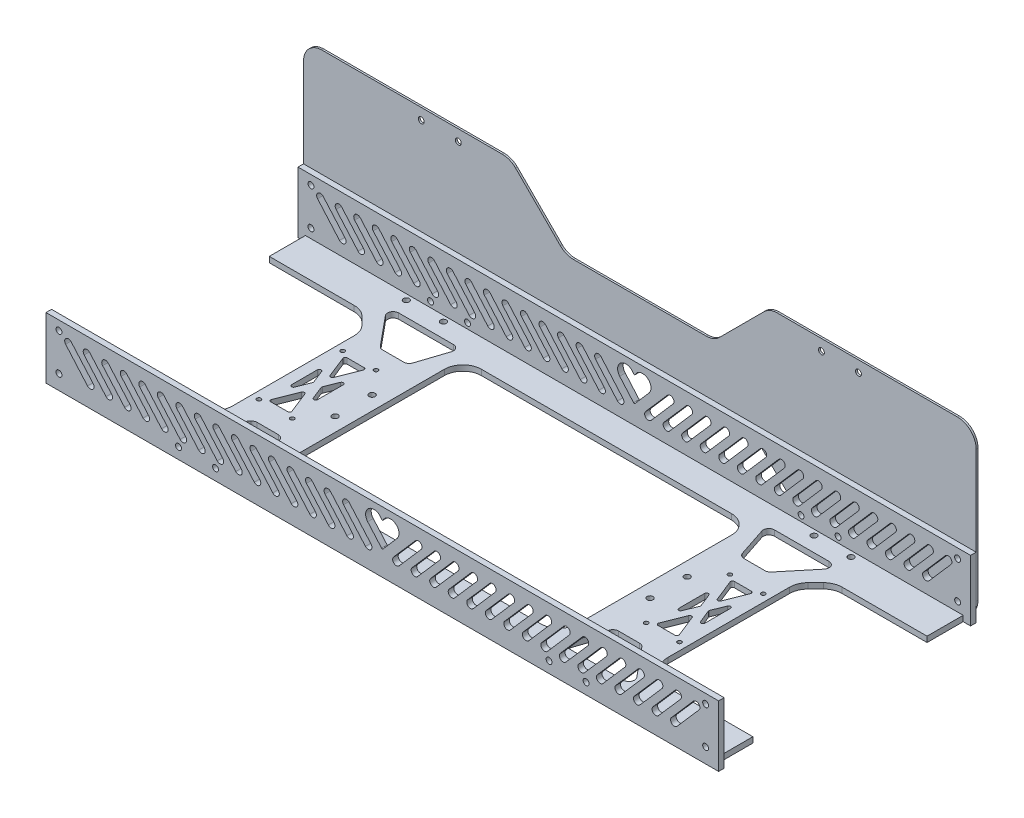
from build123d import *

# Parameters (mm, degrees)
SKETCH_1_W          = 355
SKETCH_1_H          = 133
SKETCH_1_R          = 1.6
EXTRUDE_1_DEPTH     = 3
SKETCH_2_W          = 363
SKETCH_2_H          = 33
SKETCH_2_R          = 1.6
EXTRUDE_2_DEPTH     = 3
SKETCH_3_R          = 1.6
SKETCH_3_R_2        = 1.1
CUT_EXTRUDE_1_DEPTH = 10
FILLET_1_R          = 10
CUT_EXTRUDE_2_DEPTH = 231.98105983
CUT_EXTRUDE_3_DEPTH = 10
SKETCH_7_R          = 1.6
EXTRUDE_3_DEPTH     = 1
FILLET_2_R          = 10


with BuildPart() as part:
    # 草图1 → 凸台-拉伸1 (new body)
    with BuildSketch(Plane(origin=(0, 0, 0), x_dir=(1, 0, 0), z_dir=(0, 1, 0))):
        Rectangle(SKETCH_1_W, SKETCH_1_H)
        with Locations(Location((-120, -63.5, 0), (0, 0, 270))):
            Circle(SKETCH_1_R, mode=Mode.SUBTRACT)
        with Locations(Location((120, -63.5, 0), (0, 0, 90))):
            Circle(SKETCH_1_R, mode=Mode.SUBTRACT)
        with Locations(Location((-100, -63.5, 0), (0, 0, 270))):
            Circle(SKETCH_1_R, mode=Mode.SUBTRACT)
        with Locations(Location((100, -63.5, 0), (0, 0, 90))):
            Circle(SKETCH_1_R, mode=Mode.SUBTRACT)
        with Locations(Location((100, 63.5, 0), (0, 0, 270))):
            Circle(SKETCH_1_R, mode=Mode.SUBTRACT)
        with Locations(Location((-100, 63.5, 0), (0, 0, 90))):
            Circle(SKETCH_1_R, mode=Mode.SUBTRACT)
        with Locations(Location((120, 63.5, 0), (0, 0, 270))):
            Circle(SKETCH_1_R, mode=Mode.SUBTRACT)
        with Locations(Location((-120, 63.5, 0), (0, 0, 90))):
            Circle(SKETCH_1_R, mode=Mode.SUBTRACT)
    extrude(amount=EXTRUDE_1_DEPTH)

    # 草图3 → 切除-拉伸1 (cut)
    with BuildSketch(Plane(origin=(0, 3, 0), x_dir=(1, 0, 0), z_dir=(0, 1, 0))):
        with Locations(Location((-85, 10, 0), (0, 0, 270))):
            Circle(SKETCH_3_R)
        with Locations(Location((-85, -10, 0), (0, 0, 270))):
            Circle(SKETCH_3_R)
        with Locations(Location((85, -10, 0), (0, 0, 90))):
            Circle(SKETCH_3_R)
        with Locations(Location((85, 10, 0), (0, 0, 90))):
            Circle(SKETCH_3_R)
        with Locations(Location((-113.5, 22.6, 0), (0, 0, 270))):
            Circle(SKETCH_3_R_2)
        with Locations(Location((-95.5, 22.6, 0), (0, 0, 270))):
            Circle(SKETCH_3_R_2)
        with Locations(Location((-113.5, -22.6, 0), (0, 0, 270))):
            Circle(SKETCH_3_R_2)
        with Locations(Location((-95.5, -22.6, 0), (0, 0, 270))):
            Circle(SKETCH_3_R_2)
        with Locations(Location((95.5, -22.6, 0), (0, 0, 90))):
            Circle(SKETCH_3_R_2)
        with Locations(Location((113.5, -22.6, 0), (0, 0, 90))):
            Circle(SKETCH_3_R_2)
        with Locations(Location((95.5, 22.6, 0), (0, 0, 90))):
            Circle(SKETCH_3_R_2)
        with Locations(Location((113.5, 22.6, 0), (0, 0, 90))):
            Circle(SKETCH_3_R_2)
        Polygon((-177.5, 47), (-127.5, 47), (-117.5, 37), (-117.5, -37), (-127.5, -47), (-177.5, -47), align=None)
        Polygon((177.5, 47), (127.5, 47), (117.5, 37), (117.5, -37), (127.5, -47), (177.5, -47), align=None)
        with BuildLine():
            Line((-67.5, -51.5), (67.5, -51.5))
            ThreePointArc((67.5, -51.5), (74.571067812, -48.571067812), (77.5, -41.5))
            Line((77.5, -41.5), (77.5, 41.5))
            ThreePointArc((77.5, 41.5), (74.571067812, 48.571067812), (67.5, 51.5))
            Line((67.5, 51.5), (-67.5, 51.5))
            ThreePointArc((-67.5, 51.5), (-74.571067812, 48.571067812), (-77.5, 41.5))
            Line((-77.5, 41.5), (-77.5, -41.5))
            ThreePointArc((-77.5, -41.5), (-74.571067812, -48.571067812), (-67.5, -51.5))
        make_face()
    extrude(amount=-CUT_EXTRUDE_1_DEPTH, mode=Mode.SUBTRACT)

    # 圆角1
    fillet_1_edges = [part.edges().sort_by_distance(p)[0] for p in [
        (127.5, 1.5, 47),
        (117.5, 1.5, 37),
        (117.5, 1.5, -37),
        (127.5, 1.5, -47),
        (-127.5, 1.5, -47),
        (-117.5, 1.5, -37),
        (-117.5, 1.5, 37),
        (-127.5, 1.5, 47),
    ]]
    fillet(fillet_1_edges, radius=FILLET_1_R)

    # 草图6 → 切除-拉伸3 (cut)
    with BuildSketch(Plane(origin=(0, 3, 0), x_dir=(1, 0, 0), z_dir=(0, 1, 0))):
        with BuildLine():
            Line((-109.076179073, -20.6), (-99.923820927, -20.6))
            ThreePointArc((-99.923820927, -20.6), (-99.096181899, -20.161260758), (-98.99477831, -19.230027276))
            Line((-98.99477831, -19.230027276), (-103.570957383, -7.73873316))
            ThreePointArc((-103.570957383, -7.73873316), (-104.5, -7.108705884), (-105.429042617, -7.73873316))
            Line((-105.429042617, -7.73873316), (-110.00522169, -19.230027276))
            ThreePointArc((-110.00522169, -19.230027276), (-109.903818101, -20.161260758), (-109.076179073, -20.6))
        make_face()
        with BuildLine():
            Line((-111.5, -6.957960783), (-111.5, 6.957960783))
            ThreePointArc((-111.5, 6.957960783), (-110.688357882, 7.94006124), (-109.570957383, 7.327933506))
            Line((-109.570957383, 7.327933506), (-106.800088045, 0.369972724))
            ThreePointArc((-106.800088045, 0.369972724), (-106.729130662, 0), (-106.800088045, -0.369972724))
            Line((-106.800088045, -0.369972724), (-109.570957383, -7.327933506))
            ThreePointArc((-109.570957383, -7.327933506), (-110.688357882, -7.94006124), (-111.5, -6.957960783))
        make_face()
        with BuildLine():
            Line((-103.570957383, 7.73873316), (-98.99477831, 19.230027276))
            ThreePointArc((-98.99477831, 19.230027276), (-99.096181899, 20.161260758), (-99.923820927, 20.6))
            Line((-99.923820927, 20.6), (-109.076179073, 20.6))
            ThreePointArc((-109.076179073, 20.6), (-109.903818101, 20.161260758), (-110.00522169, 19.230027276))
            Line((-110.00522169, 19.230027276), (-105.429042617, 7.73873316))
            ThreePointArc((-105.429042617, 7.73873316), (-104.5, 7.108705884), (-103.570957383, 7.73873316))
        make_face()
        with BuildLine():
            Line((-102.199911955, 0.369972724), (-99.429042617, 7.327933506))
            ThreePointArc((-99.429042617, 7.327933506), (-98.311642118, 7.94006124), (-97.5, 6.957960783))
            Line((-97.5, 6.957960783), (-97.5, -6.957960783))
            ThreePointArc((-97.5, -6.957960783), (-98.311642118, -7.94006124), (-99.429042617, -7.327933506))
            Line((-99.429042617, -7.327933506), (-102.199911955, -0.369972724))
            ThreePointArc((-102.199911955, -0.369972724), (-102.270869338, 0), (-102.199911955, 0.369972724))
        make_face()
        with BuildLine():
            Line((-118.443155104, 50.589304353), (-105.520807103, 34.947168729))
            ThreePointArc((-105.520807103, 34.947168729), (-104.486227323, 34.143818785), (-103.207964232, 33.857864376))
            Line((-103.207964232, 33.857864376), (-91.792035768, 33.857864376))
            ThreePointArc((-91.792035768, 33.857864376), (-90.033188953, 34.427543846), (-88.942328085, 35.920225789))
            Line((-88.942328085, 35.920225789), (-83.795600214, 51.562361412))
            ThreePointArc((-83.795600214, 51.562361412), (-84.214987367, 54.258846815), (-86.645307897, 55.5))
            Line((-86.645307897, 55.5), (-116.130312233, 55.5))
            ThreePointArc((-116.130312233, 55.5), (-118.844357824, 53.778263091), (-118.443155104, 50.589304353))
        make_face()
        with BuildLine():
            Line((-103.207964232, -33.857864376), (-91.792035768, -33.857864376))
            ThreePointArc((-91.792035768, -33.857864376), (-90.033188953, -34.427543846), (-88.942328085, -35.920225789))
            Line((-88.942328085, -35.920225789), (-83.795600214, -51.562361412))
            ThreePointArc((-83.795600214, -51.562361412), (-84.214987367, -54.258846815), (-86.645307897, -55.5))
            Line((-86.645307897, -55.5), (-116.130312233, -55.5))
            ThreePointArc((-116.130312233, -55.5), (-118.844357824, -53.778263091), (-118.443155104, -50.589304353))
            Line((-118.443155104, -50.589304353), (-105.520807103, -34.947168729))
            ThreePointArc((-105.520807103, -34.947168729), (-104.486227323, -34.143818785), (-103.207964232, -33.857864376))
        make_face()
        with BuildLine():
            Line((118.443155104, -50.589304353), (105.520807103, -34.947168729))
            ThreePointArc((105.520807103, -34.947168729), (104.486227323, -34.143818785), (103.207964232, -33.857864376))
            Line((103.207964232, -33.857864376), (91.792035768, -33.857864376))
            ThreePointArc((91.792035768, -33.857864376), (90.033188953, -34.427543846), (88.942328085, -35.920225789))
            Line((88.942328085, -35.920225789), (83.795600214, -51.562361412))
            ThreePointArc((83.795600214, -51.562361412), (84.214987367, -54.258846815), (86.645307897, -55.5))
            Line((86.645307897, -55.5), (116.130312233, -55.5))
            ThreePointArc((116.130312233, -55.5), (118.844357824, -53.778263091), (118.443155104, -50.589304353))
        make_face()
        with BuildLine():
            Line((86.645307897, 55.5), (116.130312233, 55.5))
            ThreePointArc((116.130312233, 55.5), (118.844357824, 53.778263091), (118.443155104, 50.589304353))
            Line((118.443155104, 50.589304353), (105.520807103, 34.947168729))
            ThreePointArc((105.520807103, 34.947168729), (104.486227323, 34.143818785), (103.207964232, 33.857864376))
            Line((103.207964232, 33.857864376), (91.792035768, 33.857864376))
            ThreePointArc((91.792035768, 33.857864376), (90.033188953, 34.427543846), (88.942328085, 35.920225789))
            Line((88.942328085, 35.920225789), (83.795600214, 51.562361412))
            ThreePointArc((83.795600214, 51.562361412), (84.214987367, 54.258846815), (86.645307897, 55.5))
        make_face()
        with BuildLine():
            Line((103.570957383, -7.73873316), (98.99477831, -19.230027276))
            ThreePointArc((98.99477831, -19.230027276), (99.096181899, -20.161260758), (99.923820927, -20.6))
            Line((99.923820927, -20.6), (109.076179073, -20.6))
            ThreePointArc((109.076179073, -20.6), (109.903818101, -20.161260758), (110.00522169, -19.230027276))
            Line((110.00522169, -19.230027276), (105.429042617, -7.73873316))
            ThreePointArc((105.429042617, -7.73873316), (104.5, -7.108705884), (103.570957383, -7.73873316))
        make_face()
        with BuildLine():
            Line((97.5, -6.957960783), (97.5, 6.957960783))
            ThreePointArc((97.5, 6.957960783), (98.311642118, 7.94006124), (99.429042617, 7.327933506))
            Line((99.429042617, 7.327933506), (102.199911955, 0.369972724))
            ThreePointArc((102.199911955, 0.369972724), (102.270869338, 0), (102.199911955, -0.369972724))
            Line((102.199911955, -0.369972724), (99.429042617, -7.327933506))
            ThreePointArc((99.429042617, -7.327933506), (98.311642118, -7.94006124), (97.5, -6.957960783))
        make_face()
        with BuildLine():
            Line((109.076179073, 20.6), (99.923820927, 20.6))
            ThreePointArc((99.923820927, 20.6), (99.096181899, 20.161260758), (98.99477831, 19.230027276))
            Line((98.99477831, 19.230027276), (103.570957383, 7.73873316))
            ThreePointArc((103.570957383, 7.73873316), (104.5, 7.108705884), (105.429042617, 7.73873316))
            Line((105.429042617, 7.73873316), (110.00522169, 19.230027276))
            ThreePointArc((110.00522169, 19.230027276), (109.903818101, 20.161260758), (109.076179073, 20.6))
        make_face()
        with BuildLine():
            Line((109.570957383, -7.327933506), (106.800088045, -0.369972724))
            ThreePointArc((106.800088045, -0.369972724), (106.729130662, 0), (106.800088045, 0.369972724))
            Line((106.800088045, 0.369972724), (109.570957383, 7.327933506))
            ThreePointArc((109.570957383, 7.327933506), (110.688357882, 7.94006124), (111.5, 6.957960783))
            Line((111.5, 6.957960783), (111.5, -6.957960783))
            ThreePointArc((111.5, -6.957960783), (110.688357882, -7.94006124), (109.570957383, -7.327933506))
        make_face()
    extrude(amount=-CUT_EXTRUDE_3_DEPTH, mode=Mode.SUBTRACT)


with BuildPart() as body_2:
    # 草图2 → 凸台-拉伸2 (new body)
    with BuildSketch(Plane.XY.offset(66.5)):
        with Locations((0, 16.5)):
            Rectangle(SKETCH_2_W, SKETCH_2_H)
        with Locations((-174.5, 28)):
            Circle(SKETCH_2_R, mode=Mode.SUBTRACT)
        with Locations(Location((174.5, 28, 0), (0, 0, 180))):
            Circle(SKETCH_2_R, mode=Mode.SUBTRACT)
        with Locations((-174.5, 8)):
            Circle(SKETCH_2_R, mode=Mode.SUBTRACT)
        with Locations(Location((174.5, 8, 0), (0, 0, 180))):
            Circle(SKETCH_2_R, mode=Mode.SUBTRACT)
        with Locations((-110, 6)):
            Circle(SKETCH_2_R, mode=Mode.SUBTRACT)
        with Locations(Location((110, 6, 0), (0, 0, 180))):
            Circle(SKETCH_2_R, mode=Mode.SUBTRACT)
        with Locations((-90, 6)):
            Circle(SKETCH_2_R, mode=Mode.SUBTRACT)
        with Locations(Location((90, 6, 0), (0, 0, 180))):
            Circle(SKETCH_2_R, mode=Mode.SUBTRACT)
    extrude(amount=EXTRUDE_2_DEPTH)


with BuildPart() as body_3:
    # 镜向1: mirrored copy
    add(body_2.part.mirror(Plane.XY))


with BuildPart() as cut_extrude_2_tool:
    # 草图4 → 切除-拉伸2 (new, through all)
    with BuildSketch(Plane.XY.offset(69.5)):
        with BuildLine():
            Line((-167.910958904, 26.095890411), (-156.075342466, 12.534246575))
            ThreePointArc((-156.075342466, 12.534246575), (-156.267123288, 9.712328767), (-159.089041096, 9.904109589))
            Line((-159.089041096, 9.904109589), (-170.924657534, 23.465753425))
            ThreePointArc((-170.924657534, 23.465753425), (-170.732876712, 26.287671233), (-167.910958904, 26.095890411))
        make_face()
        with BuildLine():
            Line((-157.910958904, 26.095890411), (-146.075342466, 12.534246575))
            ThreePointArc((-146.075342466, 12.534246575), (-146.267123288, 9.712328767), (-149.089041096, 9.904109589))
            Line((-149.089041096, 9.904109589), (-160.924657534, 23.465753425))
            ThreePointArc((-160.924657534, 23.465753425), (-160.732876712, 26.287671233), (-157.910958904, 26.095890411))
        make_face()
        with BuildLine():
            Line((-147.910958904, 26.095890411), (-136.075342466, 12.534246575))
            ThreePointArc((-136.075342466, 12.534246575), (-136.267123288, 9.712328767), (-139.089041096, 9.904109589))
            Line((-139.089041096, 9.904109589), (-150.924657534, 23.465753425))
            ThreePointArc((-150.924657534, 23.465753425), (-150.732876712, 26.287671233), (-147.910958904, 26.095890411))
        make_face()
        with BuildLine():
            Line((-137.910958904, 26.095890411), (-126.075342466, 12.534246575))
            ThreePointArc((-126.075342466, 12.534246575), (-126.267123288, 9.712328767), (-129.089041096, 9.904109589))
            Line((-129.089041096, 9.904109589), (-140.924657534, 23.465753425))
            ThreePointArc((-140.924657534, 23.465753425), (-140.732876712, 26.287671233), (-137.910958904, 26.095890411))
        make_face()
        with BuildLine():
            Line((-127.910958904, 26.095890411), (-116.075342466, 12.534246575))
            ThreePointArc((-116.075342466, 12.534246575), (-116.267123288, 9.712328767), (-119.089041096, 9.904109589))
            Line((-119.089041096, 9.904109589), (-130.924657534, 23.465753425))
            ThreePointArc((-130.924657534, 23.465753425), (-130.732876712, 26.287671233), (-127.910958904, 26.095890411))
        make_face()
        with BuildLine():
            Line((-117.910958904, 26.095890411), (-106.075342466, 12.534246575))
            ThreePointArc((-106.075342466, 12.534246575), (-106.267123288, 9.712328767), (-109.089041096, 9.904109589))
            Line((-109.089041096, 9.904109589), (-120.924657534, 23.465753425))
            ThreePointArc((-120.924657534, 23.465753425), (-120.732876712, 26.287671233), (-117.910958904, 26.095890411))
        make_face()
        with BuildLine():
            Line((-107.910958904, 26.095890411), (-96.075342466, 12.534246575))
            ThreePointArc((-96.075342466, 12.534246575), (-96.267123288, 9.712328767), (-99.089041096, 9.904109589))
            Line((-99.089041096, 9.904109589), (-110.924657534, 23.465753425))
            ThreePointArc((-110.924657534, 23.465753425), (-110.732876712, 26.287671233), (-107.910958904, 26.095890411))
        make_face()
        with BuildLine():
            Line((-97.910958904, 26.095890411), (-86.075342466, 12.534246575))
            ThreePointArc((-86.075342466, 12.534246575), (-86.267123288, 9.712328767), (-89.089041096, 9.904109589))
            Line((-89.089041096, 9.904109589), (-100.924657534, 23.465753425))
            ThreePointArc((-100.924657534, 23.465753425), (-100.732876712, 26.287671233), (-97.910958904, 26.095890411))
        make_face()
        with BuildLine():
            Line((-87.910958904, 26.095890411), (-76.075342466, 12.534246575))
            ThreePointArc((-76.075342466, 12.534246575), (-76.267123288, 9.712328767), (-79.089041096, 9.904109589))
            Line((-79.089041096, 9.904109589), (-90.924657534, 23.465753425))
            ThreePointArc((-90.924657534, 23.465753425), (-90.732876712, 26.287671233), (-87.910958904, 26.095890411))
        make_face()
        with BuildLine():
            Line((-77.910958904, 26.095890411), (-66.075342466, 12.534246575))
            ThreePointArc((-66.075342466, 12.534246575), (-66.267123288, 9.712328767), (-69.089041096, 9.904109589))
            Line((-69.089041096, 9.904109589), (-80.924657534, 23.465753425))
            ThreePointArc((-80.924657534, 23.465753425), (-80.732876712, 26.287671233), (-77.910958904, 26.095890411))
        make_face()
        with BuildLine():
            Line((-67.910958904, 26.095890411), (-56.075342466, 12.534246575))
            ThreePointArc((-56.075342466, 12.534246575), (-56.267123288, 9.712328767), (-59.089041096, 9.904109589))
            Line((-59.089041096, 9.904109589), (-70.924657534, 23.465753425))
            ThreePointArc((-70.924657534, 23.465753425), (-70.732876712, 26.287671233), (-67.910958904, 26.095890411))
        make_face()
        with BuildLine():
            Line((-57.910958904, 26.095890411), (-46.075342466, 12.534246575))
            ThreePointArc((-46.075342466, 12.534246575), (-46.267123288, 9.712328767), (-49.089041096, 9.904109589))
            Line((-49.089041096, 9.904109589), (-60.924657534, 23.465753425))
            ThreePointArc((-60.924657534, 23.465753425), (-60.732876712, 26.287671233), (-57.910958904, 26.095890411))
        make_face()
        with BuildLine():
            Line((-47.910958904, 26.095890411), (-36.075342466, 12.534246575))
            ThreePointArc((-36.075342466, 12.534246575), (-36.267123288, 9.712328767), (-39.089041096, 9.904109589))
            Line((-39.089041096, 9.904109589), (-50.924657534, 23.465753425))
            ThreePointArc((-50.924657534, 23.465753425), (-50.732876712, 26.287671233), (-47.910958904, 26.095890411))
        make_face()
        with BuildLine():
            Line((-37.910958904, 26.095890411), (-26.075342466, 12.534246575))
            ThreePointArc((-26.075342466, 12.534246575), (-26.267123288, 9.712328767), (-29.089041096, 9.904109589))
            Line((-29.089041096, 9.904109589), (-40.924657534, 23.465753425))
            ThreePointArc((-40.924657534, 23.465753425), (-40.732876712, 26.287671233), (-37.910958904, 26.095890411))
        make_face()
        with BuildLine():
            Line((-27.910958904, 26.095890411), (-16.075342466, 12.534246575))
            ThreePointArc((-16.075342466, 12.534246575), (-16.267123288, 9.712328767), (-19.089041096, 9.904109589))
            Line((-19.089041096, 9.904109589), (-30.924657534, 23.465753425))
            ThreePointArc((-30.924657534, 23.465753425), (-30.732876712, 26.287671233), (-27.910958904, 26.095890411))
        make_face()
        with BuildLine():
            Line((-17.910958904, 26.095890411), (-6.075342466, 12.534246575))
            ThreePointArc((-6.075342466, 12.534246575), (-6.267123288, 9.712328767), (-9.089041096, 9.904109589))
            Line((-9.089041096, 9.904109589), (-20.924657534, 23.465753425))
            ThreePointArc((-20.924657534, 23.465753425), (-20.732876712, 26.287671233), (-17.910958904, 26.095890411))
        make_face()
        with BuildLine():
            Line((167.910958904, 26.095890411), (156.075342466, 12.534246575))
            ThreePointArc((156.075342466, 12.534246575), (156.267123288, 9.712328767), (159.089041096, 9.904109589))
            Line((159.089041096, 9.904109589), (170.924657534, 23.465753425))
            ThreePointArc((170.924657534, 23.465753425), (170.732876712, 26.287671233), (167.910958904, 26.095890411))
        make_face()
        with BuildLine():
            Line((157.910958904, 26.095890411), (146.075342466, 12.534246575))
            ThreePointArc((146.075342466, 12.534246575), (146.267123288, 9.712328767), (149.089041096, 9.904109589))
            Line((149.089041096, 9.904109589), (160.924657534, 23.465753425))
            ThreePointArc((160.924657534, 23.465753425), (160.732876712, 26.287671233), (157.910958904, 26.095890411))
        make_face()
        with BuildLine():
            Line((147.910958904, 26.095890411), (136.075342466, 12.534246575))
            ThreePointArc((136.075342466, 12.534246575), (136.267123288, 9.712328767), (139.089041096, 9.904109589))
            Line((139.089041096, 9.904109589), (150.924657534, 23.465753425))
            ThreePointArc((150.924657534, 23.465753425), (150.732876712, 26.287671233), (147.910958904, 26.095890411))
        make_face()
        with BuildLine():
            Line((137.910958904, 26.095890411), (126.075342466, 12.534246575))
            ThreePointArc((126.075342466, 12.534246575), (126.267123288, 9.712328767), (129.089041096, 9.904109589))
            Line((129.089041096, 9.904109589), (140.924657534, 23.465753425))
            ThreePointArc((140.924657534, 23.465753425), (140.732876712, 26.287671233), (137.910958904, 26.095890411))
        make_face()
        with BuildLine():
            Line((127.910958904, 26.095890411), (116.075342466, 12.534246575))
            ThreePointArc((116.075342466, 12.534246575), (116.267123288, 9.712328767), (119.089041096, 9.904109589))
            Line((119.089041096, 9.904109589), (130.924657534, 23.465753425))
            ThreePointArc((130.924657534, 23.465753425), (130.732876712, 26.287671233), (127.910958904, 26.095890411))
        make_face()
        with BuildLine():
            Line((117.910958904, 26.095890411), (106.075342466, 12.534246575))
            ThreePointArc((106.075342466, 12.534246575), (106.267123288, 9.712328767), (109.089041096, 9.904109589))
            Line((109.089041096, 9.904109589), (120.924657534, 23.465753425))
            ThreePointArc((120.924657534, 23.465753425), (120.732876712, 26.287671233), (117.910958904, 26.095890411))
        make_face()
        with BuildLine():
            Line((107.910958904, 26.095890411), (96.075342466, 12.534246575))
            ThreePointArc((96.075342466, 12.534246575), (96.267123288, 9.712328767), (99.089041096, 9.904109589))
            Line((99.089041096, 9.904109589), (110.924657534, 23.465753425))
            ThreePointArc((110.924657534, 23.465753425), (110.732876712, 26.287671233), (107.910958904, 26.095890411))
        make_face()
        with BuildLine():
            Line((97.910958904, 26.095890411), (86.075342466, 12.534246575))
            ThreePointArc((86.075342466, 12.534246575), (86.267123288, 9.712328767), (89.089041096, 9.904109589))
            Line((89.089041096, 9.904109589), (100.924657534, 23.465753425))
            ThreePointArc((100.924657534, 23.465753425), (100.732876712, 26.287671233), (97.910958904, 26.095890411))
        make_face()
        with BuildLine():
            Line((87.910958904, 26.095890411), (76.075342466, 12.534246575))
            ThreePointArc((76.075342466, 12.534246575), (76.267123288, 9.712328767), (79.089041096, 9.904109589))
            Line((79.089041096, 9.904109589), (90.924657534, 23.465753425))
            ThreePointArc((90.924657534, 23.465753425), (90.732876712, 26.287671233), (87.910958904, 26.095890411))
        make_face()
        with BuildLine():
            Line((77.910958904, 26.095890411), (66.075342466, 12.534246575))
            ThreePointArc((66.075342466, 12.534246575), (66.267123288, 9.712328767), (69.089041096, 9.904109589))
            Line((69.089041096, 9.904109589), (80.924657534, 23.465753425))
            ThreePointArc((80.924657534, 23.465753425), (80.732876712, 26.287671233), (77.910958904, 26.095890411))
        make_face()
        with BuildLine():
            Line((67.910958904, 26.095890411), (56.075342466, 12.534246575))
            ThreePointArc((56.075342466, 12.534246575), (56.267123288, 9.712328767), (59.089041096, 9.904109589))
            Line((59.089041096, 9.904109589), (70.924657534, 23.465753425))
            ThreePointArc((70.924657534, 23.465753425), (70.732876712, 26.287671233), (67.910958904, 26.095890411))
        make_face()
        with BuildLine():
            Line((57.910958904, 26.095890411), (46.075342466, 12.534246575))
            ThreePointArc((46.075342466, 12.534246575), (46.267123288, 9.712328767), (49.089041096, 9.904109589))
            Line((49.089041096, 9.904109589), (60.924657534, 23.465753425))
            ThreePointArc((60.924657534, 23.465753425), (60.732876712, 26.287671233), (57.910958904, 26.095890411))
        make_face()
        with BuildLine():
            Line((47.910958904, 26.095890411), (36.075342466, 12.534246575))
            ThreePointArc((36.075342466, 12.534246575), (36.267123288, 9.712328767), (39.089041096, 9.904109589))
            Line((39.089041096, 9.904109589), (50.924657534, 23.465753425))
            ThreePointArc((50.924657534, 23.465753425), (50.732876712, 26.287671233), (47.910958904, 26.095890411))
        make_face()
        with BuildLine():
            Line((37.910958904, 26.095890411), (26.075342466, 12.534246575))
            ThreePointArc((26.075342466, 12.534246575), (26.267123288, 9.712328767), (29.089041096, 9.904109589))
            Line((29.089041096, 9.904109589), (40.924657534, 23.465753425))
            ThreePointArc((40.924657534, 23.465753425), (40.732876712, 26.287671233), (37.910958904, 26.095890411))
        make_face()
        with BuildLine():
            Line((27.910958904, 26.095890411), (16.075342466, 12.534246575))
            ThreePointArc((16.075342466, 12.534246575), (16.267123288, 9.712328767), (19.089041096, 9.904109589))
            Line((19.089041096, 9.904109589), (30.924657534, 23.465753425))
            ThreePointArc((30.924657534, 23.465753425), (30.732876712, 26.287671233), (27.910958904, 26.095890411))
        make_face()
        with BuildLine():
            Line((17.910958904, 26.095890411), (6.075342466, 12.534246575))
            ThreePointArc((6.075342466, 12.534246575), (6.267123288, 9.712328767), (9.089041096, 9.904109589))
            Line((9.089041096, 9.904109589), (20.924657534, 23.465753425))
            ThreePointArc((20.924657534, 23.465753425), (20.732876712, 26.287671233), (17.910958904, 26.095890411))
        make_face()
        with BuildLine():
            Line((-0.376712329, 13.431649543), (-7.890410959, 22.04109589))
            ThreePointArc((-7.890410959, 22.04109589), (-6.982210649, 28.753482422), (-0.45, 26.961504525))
            ThreePointArc((-0.45, 26.961504525), (0, 26.679449472), (0.45, 26.961504525))
            ThreePointArc((0.45, 26.961504525), (6.982210649, 28.753482422), (7.890410959, 22.04109589))
            Line((7.890410959, 22.04109589), (0.376712329, 13.431649543))
            ThreePointArc((0.376712329, 13.431649543), (0, 13.260416667), (-0.376712329, 13.431649543))
        make_face()
    extrude(amount=-CUT_EXTRUDE_2_DEPTH)


with BuildPart() as body_2_1:
    add(body_2.part)

    # 切除-拉伸2: cut by cut_extrude_2_tool
    add(cut_extrude_2_tool.part, mode=Mode.SUBTRACT)


with BuildPart() as body_3_1:
    add(body_3.part)

    # 切除-拉伸2: cut by cut_extrude_2_tool
    add(cut_extrude_2_tool.part, mode=Mode.SUBTRACT)


with BuildPart() as body_4:
    # 草图7 → 凸台-拉伸3 (new body)
    with BuildSketch(Plane.XY.offset(-69.5)):
        Polygon((-181.5, 0), (-181.5, 91.15), (-70, 91.15), (-40, 61.15), (40, 61.15), (70, 91.15), (181.5, 91.15), (181.5, 0), (89.5, 0), (58.5, 31), (-58.5, 31), (-89.5, 0), align=None)
        with Locations((-174.5, 28)):
            Circle(SKETCH_7_R, mode=Mode.SUBTRACT)
        with Locations((-174.5, 8)):
            Circle(SKETCH_7_R, mode=Mode.SUBTRACT)
        with Locations((-110, 6)):
            Circle(SKETCH_7_R, mode=Mode.SUBTRACT)
        with Locations((-90, 6)):
            Circle(SKETCH_7_R, mode=Mode.SUBTRACT)
        with Locations((90, 6)):
            Circle(SKETCH_7_R, mode=Mode.SUBTRACT)
        with Locations((110, 6)):
            Circle(SKETCH_7_R, mode=Mode.SUBTRACT)
        with Locations((174.5, 8)):
            Circle(SKETCH_7_R, mode=Mode.SUBTRACT)
        with Locations((174.5, 28)):
            Circle(SKETCH_7_R, mode=Mode.SUBTRACT)
        with Locations((118, 85.15)):
            Circle(SKETCH_7_R, mode=Mode.SUBTRACT)
        with Locations((98, 85.15)):
            Circle(SKETCH_7_R, mode=Mode.SUBTRACT)
        with Locations(Location((-98, 85.15, 0), (0, 0, 180))):
            Circle(SKETCH_7_R, mode=Mode.SUBTRACT)
        with Locations(Location((-118, 85.15, 0), (0, 0, 180))):
            Circle(SKETCH_7_R, mode=Mode.SUBTRACT)
    extrude(amount=-EXTRUDE_3_DEPTH)

    # 圆角2
    fillet_2_edges = [body_4.edges().sort_by_distance(p)[0] for p in [
        (-181.5, 0, -70),
        (-181.5, 91.15, -70),
        (-70, 91.15, -70),
        (-40, 61.15, -70),
        (40, 61.15, -70),
        (70, 91.15, -70),
        (181.5, 91.15, -70),
        (181.5, 0, -70),
        (89.5, 0, -70),
        (58.5, 31, -70),
        (-58.5, 31, -70),
        (-89.5, 0, -70),
    ]]
    fillet(fillet_2_edges, radius=FILLET_2_R)


solid = Compound([part.part, body_2_1.part, body_3_1.part, body_4.part])
